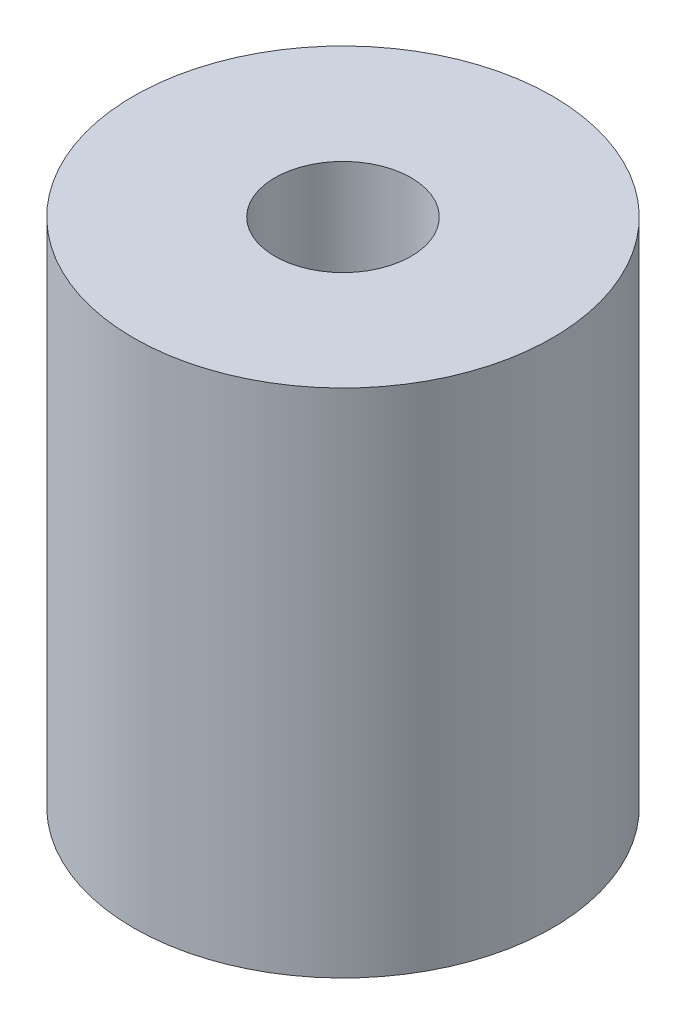
from build123d import *

# Parameters (mm, degrees)
SKETCH_1_W = 8.3
SKETCH_1_H = 30


with BuildPart() as part:
    # 草图1 → 旋转1 (revolve)
    with BuildSketch(Plane.XY, mode=Mode.PRIVATE) as revolve_1_sk:
        with Locations((8.15, 10.747308607)):
            Rectangle(SKETCH_1_W, SKETCH_1_H)
    revolve(revolve_1_sk.sketch.rotate(Axis((0, 0, 0), (0, 1, 0)), 90), axis=Axis((0, 0, 0), (0, 1, 0)))


solid = part.part
